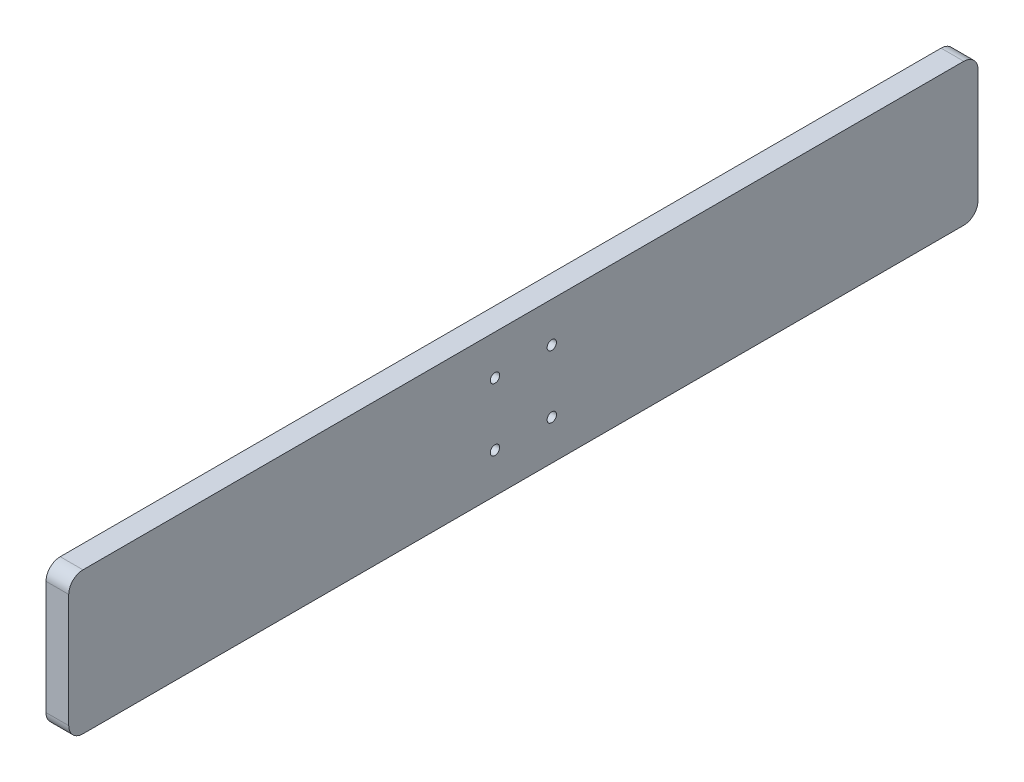
SolidWorks part; units mm, degrees
ref_plane "前视基准面" through (0, 0, 0) normal (0, 0, 1) x (1, 0, 0)
ref_plane "上视基准面" through (0, 0, 0) normal (0, 1, 0) x (1, 0, 0)
ref_plane "右视基准面" through (0, 0, 0) normal (1, 0, 0) x (0, 0, -1)
sketch "草图1" plane through (0, 0, 0) normal (1, 0, 0) x (0, 0, -1)
  line L1 (-160, 25) -> (160, 25)
  line L2 (-160, 25) -> (-160, -25)
  line L3 (-160, -25) -> (160, -25)
  line L4 (160, 25) -> (160, -25)
  line L5 (-160, 25) -> (160, -25) construction
  line L6 (-160, -25) -> (160, 25) construction
  point P0 (0, 0)
  dimension "D1" = 320
  dimension "D2" = 50
extrude "凸台-拉伸1" add sketch "草图1" along normal blind 8
hole_wizard "M4 螺纹孔1" positions "草图4" profile "草图6" tap size "M4" standard "ISO" end condition through all
sketch "草图4" plane through (0, 0, 0) normal (-1, 0, 0) x (0, 0, 1)
  line L0 (0, 0) -> (0, 25) construction
  line L1 (-160, 25) -> (160, 25) construction
  line L3 (0, 0) -> (-17.5026, 0) construction
  point P0 (-10, -11)
  point P3 (-10, 11)
  point P5 (10, -11)
  point P7 (10, 11)
  dimension "D1" = 22
  dimension "D2" = 20
sketch "草图6" plane through (0, -11, -10) normal (0, 1, 0) x (0, 0, 1)
  line L0 (0, 0) -> (0, 8)
  line L1 (0, 8) -> (1.65, 8)
  line L2 (1.65, 8) -> (1.65, 0)
  line L5 (1.65, 0) -> (0, 0)
  line L11 (0, -6.35) -> (0, 107.95) construction
  dimension "通孔螺纹孔钻头直径" = 3.3
  dimension "通孔螺纹孔钻头深度" = 8
cosmetic thread "孔螺蚊线1" parameters "D2"=4
cosmetic thread "孔螺蚊线2" parameters "D2"=4
cosmetic thread "孔螺蚊线3" parameters "D2"=4
cosmetic thread "孔螺蚊线4" parameters "D2"=4
fillet "圆角1" radius 5 4 edges at (4, 25, 160) (4, -25, 160) (4, -25, -160) (4, 25, -160)
